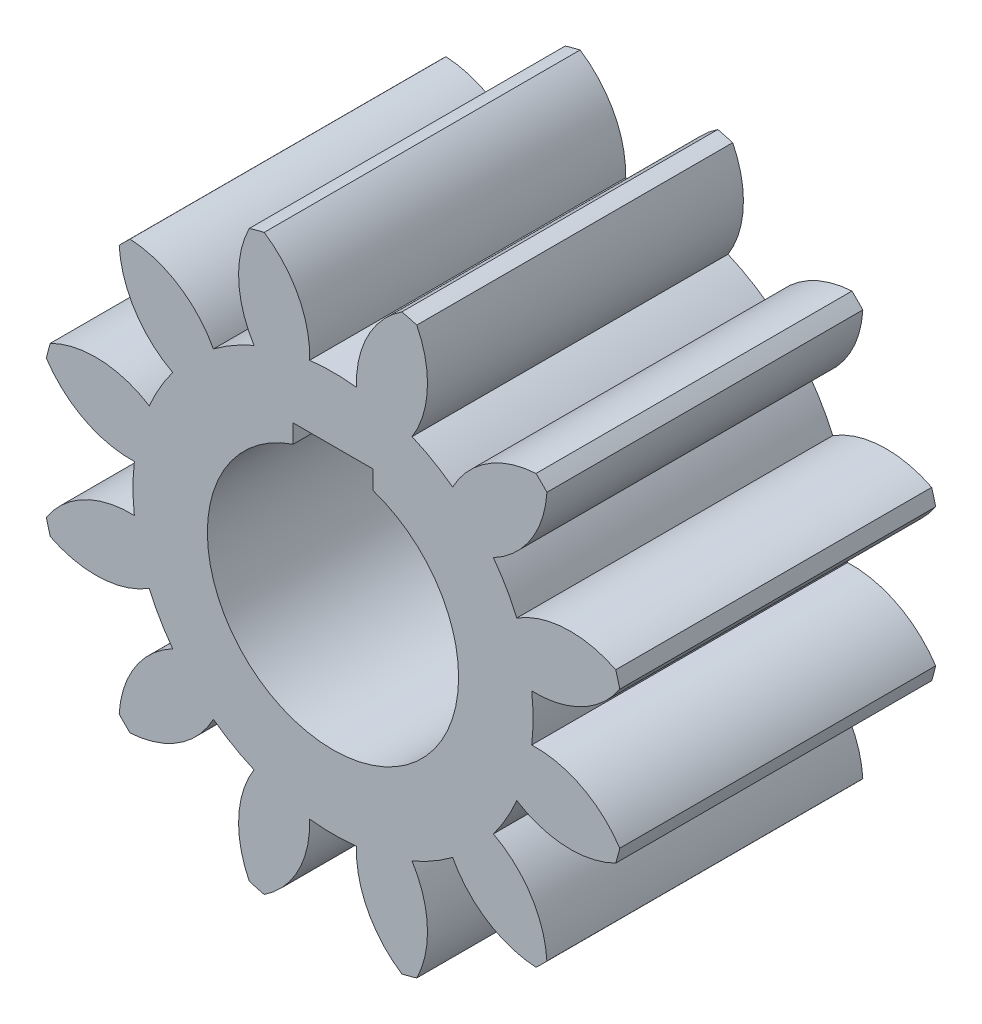
SolidWorks part; units mm, degrees
ref_plane "前视基准面" through (0, 0, 0) normal (0, 0, 1) x (1, 0, 0)
ref_plane "上视基准面" through (0, 0, 0) normal (0, 1, 0) x (1, 0, 0)
ref_plane "右视基准面" through (0, 0, 0) normal (1, 0, 0) x (0, 0, -1)
other "Configuration Table"
sketch "草图2" plane through (0, 0, 0) normal (0, 0, 1) x (1, 0, 0)
  line L0 (-0.0029, -0.0678) -> (-0.0029, 6.4684) construction
  line L1 (1.8884, 6.4684) -> (-1.8942, 6.4684) construction
  line L2 (-1.8942, 6.4684) -> (-1.8942, 5.589) construction
  line L3 (1.8884, 6.4684) -> (1.8884, 5.589) construction
  line L4 (-1.8942, 6.4684) -> (1.8884, 6.4684)
  line L5 (1.8884, 6.4684) -> (1.8884, 5.589)
  line L6 (-1.8942, 5.589) -> (-1.8942, 6.4684)
  arc A0 (-1.8942, 5.589) -> (1.8884, 5.589) centre (-0.0029, -0.0678) ccw
  arc A96 (-10.1547, 9.6375) -> (-7.6139, 5.6798) centre (-5.363, 9.9193) ccw
  arc A97 (-7.6139, 5.6798) -> (-8.7258, 3.7539) centre (0, 0) ccw
  arc A98 (-8.7258, 3.7539) -> (-13.4237, 3.9755) centre (-11.2719, -0.3151) ccw
  arc A99 (-13.4237, 3.9755) -> (-13.613, 3.2689) centre (0, 0) ccw
  arc A100 (-13.613, 3.2689) -> (-9.4337, 1.1119) centre (-9.6042, 5.9089) ccw
  arc A101 (-9.4337, 1.1119) -> (-9.4337, -1.1119) centre (0, 0) ccw
  arc A102 (-9.4337, -1.1119) -> (-13.613, -3.2689) centre (-9.6042, -5.9089) ccw
  arc A103 (-13.613, -3.2689) -> (-13.4237, -3.9755) centre (0, 0) ccw
  arc A104 (-13.4237, -3.9755) -> (-8.7258, -3.7539) centre (-11.2719, 0.3151) ccw
  arc A105 (-8.7258, -3.7539) -> (-7.6139, -5.6798) centre (0, 0) ccw
  arc A106 (-7.6139, -5.6798) -> (-10.1547, -9.6375) centre (-5.363, -9.9193) ccw
  arc A107 (-10.1547, -9.6375) -> (-9.6375, -10.1547) centre (0, 0) ccw
  arc A108 (-9.6375, -10.1547) -> (-5.6798, -7.6139) centre (-9.9193, -5.363) ccw
  arc A109 (-5.6798, -7.6139) -> (-3.7539, -8.7258) centre (0, 0) ccw
  arc A110 (-3.7539, -8.7258) -> (-3.9755, -13.4237) centre (0.3151, -11.2719) ccw
  arc A111 (-3.9755, -13.4237) -> (-3.2689, -13.613) centre (0, 0) ccw
  arc A112 (-3.2689, -13.613) -> (-1.1119, -9.4337) centre (-5.9089, -9.6042) ccw
  arc A113 (-1.1119, -9.4337) -> (1.1119, -9.4337) centre (0, 0) ccw
  arc A114 (1.1119, -9.4337) -> (3.2689, -13.613) centre (5.9089, -9.6042) ccw
  arc A115 (3.2689, -13.613) -> (3.9755, -13.4237) centre (0, 0) ccw
  arc A116 (3.9755, -13.4237) -> (3.7539, -8.7258) centre (-0.3151, -11.2719) ccw
  arc A117 (3.7539, -8.7258) -> (5.6798, -7.6139) centre (0, 0) ccw
  arc A118 (5.6798, -7.6139) -> (9.6375, -10.1547) centre (9.9193, -5.363) ccw
  arc A119 (9.6375, -10.1547) -> (10.1547, -9.6375) centre (0, 0) ccw
  arc A120 (10.1547, -9.6375) -> (7.6139, -5.6798) centre (5.363, -9.9193) ccw
  arc A121 (7.6139, -5.6798) -> (8.7258, -3.7539) centre (0, 0) ccw
  arc A122 (8.7258, -3.7539) -> (13.4237, -3.9755) centre (11.2719, 0.3151) ccw
  arc A123 (13.4237, -3.9755) -> (13.613, -3.2689) centre (0, 0) ccw
  arc A124 (13.613, -3.2689) -> (9.4337, -1.1119) centre (9.6042, -5.9089) ccw
  arc A125 (9.4337, -1.1119) -> (9.4337, 1.1119) centre (0, 0) ccw
  arc A126 (9.4337, 1.1119) -> (13.613, 3.2689) centre (9.6042, 5.9089) ccw
  arc A127 (13.613, 3.2689) -> (13.4237, 3.9755) centre (0, 0) ccw
  arc A128 (13.4237, 3.9755) -> (8.7258, 3.7539) centre (11.2719, -0.3151) ccw
  arc A129 (8.7258, 3.7539) -> (7.6139, 5.6798) centre (0, 0) ccw
  arc A130 (7.6139, 5.6798) -> (10.1547, 9.6375) centre (5.363, 9.9193) ccw
  arc A131 (10.1547, 9.6375) -> (9.6375, 10.1547) centre (0, 0) ccw
  arc A132 (9.6375, 10.1547) -> (5.6798, 7.6139) centre (9.9193, 5.363) ccw
  arc A133 (5.6798, 7.6139) -> (3.7539, 8.7258) centre (0, 0) ccw
  arc A134 (3.7539, 8.7258) -> (3.9755, 13.4237) centre (-0.3151, 11.2719) ccw
  arc A135 (3.9755, 13.4237) -> (3.2689, 13.613) centre (0, 0) ccw
  arc A136 (3.2689, 13.613) -> (1.1119, 9.4337) centre (5.9089, 9.6042) ccw
  arc A137 (1.1119, 9.4337) -> (-1.1119, 9.4337) centre (0, 0) ccw
  arc A138 (-1.1119, 9.4337) -> (-3.2689, 13.613) centre (-5.9089, 9.6042) ccw
  arc A139 (-3.2689, 13.613) -> (-3.9755, 13.4237) centre (0, 0) ccw
  arc A140 (-3.9755, 13.4237) -> (-3.7539, 8.7258) centre (0.3151, 11.2719) ccw
  arc A141 (-3.7539, 8.7258) -> (-5.6798, 7.6139) centre (0, 0) ccw
  arc A142 (-5.6798, 7.6139) -> (-9.6375, 10.1547) centre (-9.9193, 5.363) ccw
  arc A143 (-9.6375, 10.1547) -> (-10.1547, 9.6375) centre (0, 0) ccw
  point P6 (-0.0029, -6.0325)
extrude "凸台-拉伸1" add sketch "草图2" along normal blind 15
